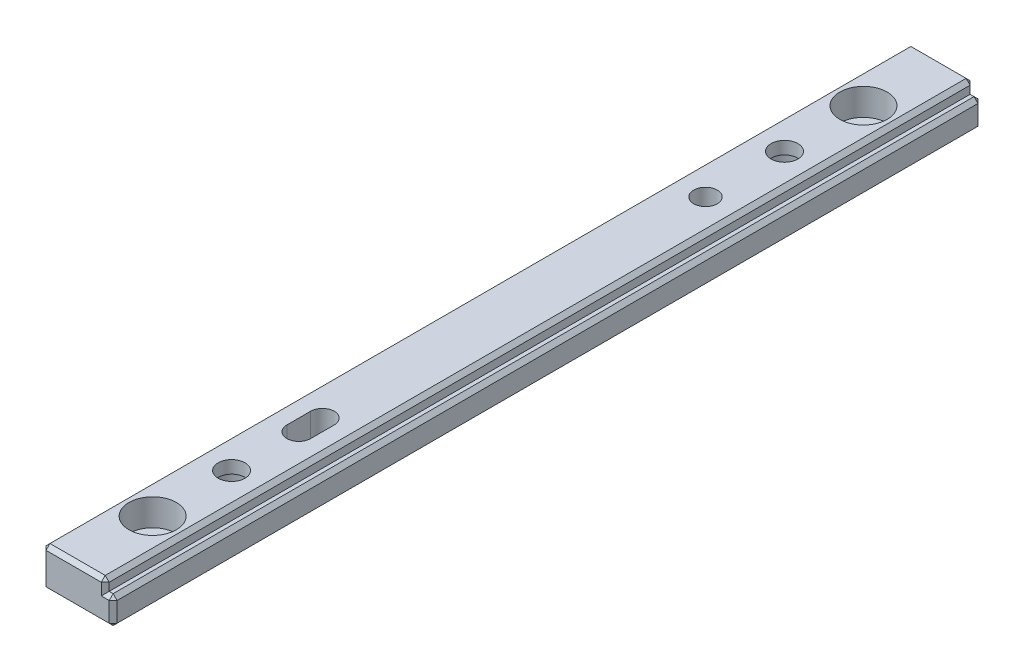
SolidWorks part; units mm, degrees
ref_plane "Front Plane" through (0, 0, 0) normal (0, 0, 1) x (1, 0, 0)
ref_plane "Top Plane" through (0, 0, 0) normal (0, 1, 0) x (1, 0, 0)
ref_plane "Right Plane" through (0, 0, 0) normal (1, 0, 0) x (0, 0, -1)
other "Configuration Table"
sketch "Sketch4" plane through (0, 0, 0) normal (0, 0, 1) x (1, 0, 0)
  line L1 (0, 0) -> (9, 0)
  line L2 (0, 0) -> (0, 3.5)
  line L3 (8, 3.5) -> (9, 3.5)
  line L4 (9, 0) -> (9, 3.5)
  line L6 (0, 3.5) -> (0, 5)
  line L7 (0, 5) -> (8, 5)
  line L8 (8, 3.5) -> (8, 5)
  dimension "D1" = 5
  dimension "D2" = 1.5
  dimension "D3" = 8
  dimension "D4" = 9
extrude "Boss-Extrude2" add sketch "Sketch4" along normal blind 110
sketch "Sketch5" plane through (0, 5, 0) normal (0, 1, 0) x (1, 0, 0)
  line L0 (0, -110) -> (0, 0) construction
  line L1 (8, 0) -> (0, 0) construction
  line L2 (8, -110) -> (0, -110) construction
  point P0 (4, -10)
  point P1 (4, -100)
  dimension "D1" = 4
  dimension "D2" = 10
  dimension "D3" = 10
  dimension "D4" = 90
hole_wizard "CBORE for M3 Slotted cheese head screws2" positions "Sketch5" profile "Sketch6" counterbore size "M3" standard "GB" end condition through all
sketch "Sketch6" plane through (4, 5, 10) normal (1, 0, 0) x (0, 0, 1)
  line L0 (0, 0) -> (0, 5)
  line L1 (0, 5) -> (1.7, 5)
  line L3 (1.7, 5) -> (1.7, 3.4)
  line L4 (1.7, 3.4) -> (3, 3.4)
  line L5 (3, 3.4) -> (3, 0)
  line L7 (3, 0) -> (0, 0)
  line L11 (0, -6.35) -> (0, 107.95) construction
  dimension "通孔孔直径" = 3.4
  dimension "通孔孔深度" = 5
  dimension "柱形沉头孔直径" = 6
  dimension "柱形沉头孔深度" = 3.4
sketch "Sketch7" plane through (0, 0, 0) normal (0, -1, 0) x (1, 0, 0)
  line L0 (0, 110) -> (0, 0) construction
  circle A0 centre (4, 100) radius 1.7 construction
  circle A1 centre (4, 10) radius 1.7 construction
  point P0 (4, 90)
  point P5 (4, 20)
  dimension "D3" = 10
  dimension "D1" = 4
  dimension "D2" = 10
  dimension "D4" = 70
hole_wizard "CBORE for M3 Slotted cheese head screws3" positions "Sketch7" profile "Sketch8" counterbore size "M3" standard "GB" end condition through all
sketch "Sketch8" plane through (4, 0, 90) normal (1, 0, 0) x (0, 0, -1)
  line L0 (0, 0) -> (0, 5)
  line L1 (0, 5) -> (1.7, 5)
  line L3 (1.7, 5) -> (1.7, 3.4)
  line L4 (1.7, 3.4) -> (3, 3.4)
  line L5 (3, 3.4) -> (3, 0)
  line L7 (3, 0) -> (0, 0)
  line L11 (0, -6.35) -> (0, 107.95) construction
  dimension "通孔孔直径" = 3.4
  dimension "通孔孔深度" = 5
  dimension "柱形沉头孔直径" = 6
  dimension "柱形沉头孔深度" = 3.4
sketch "Sketch9" plane through (0, 0, 0) normal (0, -1, 0) x (1, 0, 0)
  line L0 (0, 110) -> (0, 0) construction
  circle A0 centre (4, 90) radius 1.7 construction
  circle A1 centre (4, 20) radius 1.7 construction
  point P0 (4, 80)
  point P1 (4, 30)
  dimension "D2" = 10
  dimension "D1" = 4
  dimension "D3" = 10
  dimension "D4" = 50
hole_wizard "Ø3.0mm dowel hole1" positions "Sketch9" profile "Sketch10" hole size "Ø3.0" standard "GB" end condition through all
sketch "Sketch10" plane through (4, 0, 80) normal (1, 0, 0) x (0, 0, -1)
  line L0 (0, 0) -> (0, 5)
  line L1 (0, 5) -> (1.5, 5)
  line L2 (1.5, 5) -> (1.5, 0)
  line L5 (1.5, 0) -> (0, 0)
  line L11 (0, -6.35) -> (0, 107.95) construction
  dimension "通孔孔直径" = 3
  dimension "通孔孔深度" = 5
sketch "Sketch11" plane through (0, 0, 0) normal (0, -1, 0) x (1, 0, 0)
  line L0 (4, 78.5) -> (4, 81.5) construction
  line L1 (2.5, 78.5) -> (2.5, 81.5)
  line L2 (5.5, 78.5) -> (5.5, 81.5)
  circle A0 centre (4, 80) radius 1.5 construction
  arc A1 (2.5, 78.5) -> (5.5, 78.5) centre (4, 78.5) ccw
  arc A2 (5.5, 81.5) -> (2.5, 81.5) centre (4, 81.5) ccw
  point P5 (4, 80)
  dimension "D1" = 1.5
extrude "Cut-Extrude1" cut sketch "Sketch11" against normal through all
chamfer "Chamfer1" distance 0.5 17 edges at (9, 0, 55) (9, 3.5, 55) (9, 1.75, 0) (8.5, 3.5, 0) (8, 4.25, 0) (4, 5, 0) (4.5, 0, 0) (4, 5, 110) (0, 5, 55) (0, 2.5, 110) (0, 2.5, 0) (0, 0, 55) (4.5, 0, 110) (9, 1.75, 110) (8.5, 3.5, 110) (8, 4.25, 110) (8, 5, 55)
